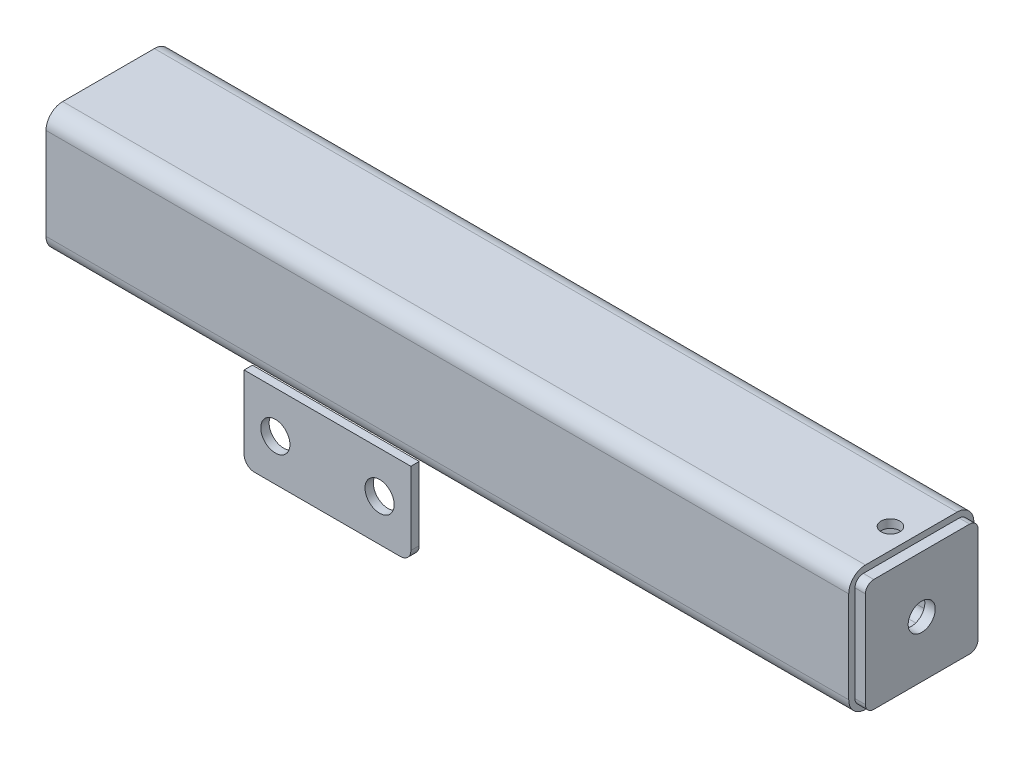
from build123d import *

# Parameters (mm, degrees)
GB_T6728_2002_60_X_60_X_4_1_DEPTH = 385
EXTRUDE_1_DEPTH                   = 5
SKETCH_4_R                        = 7
EXTRUDE_2_DEPTH                   = 4
SKETCH_5_R                        = 6.5
CUT_EXTRUDE_1_DEPTH               = 5


with BuildPart() as part:
    # Sketch1 → 冷弯空心方管gb∕t6728-2002 60 X 60 X 4(1) (new body)
    with BuildSketch(Plane.YZ):
        with BuildLine():
            Line((-22, -30), (22, -30))
            ThreePointArc((22, -30), (27.656854249, -27.656854249), (30, -22))
            Line((30, -22), (30, 22))
            ThreePointArc((30, 22), (27.656854249, 27.656854249), (22, 30))
            Line((22, 30), (-22, 30))
            ThreePointArc((-22, 30), (-27.656854249, 27.656854249), (-30, 22))
            Line((-30, 22), (-30, -22))
            ThreePointArc((-30, -22), (-27.656854249, -27.656854249), (-22, -30))
        make_face()
        with BuildLine():
            Line((-22, -26), (22, -26))
            ThreePointArc((22, -26), (24.828427125, -24.828427125), (26, -22))
            Line((26, -22), (26, 22))
            ThreePointArc((26, 22), (24.828427125, 24.828427125), (22, 26))
            Line((22, 26), (-22, 26))
            ThreePointArc((-22, 26), (-24.828427125, 24.828427125), (-26, 22))
            Line((-26, 22), (-26, -22))
            ThreePointArc((-26, -22), (-24.828427125, -24.828427125), (-22, -26))
        make_face(mode=Mode.SUBTRACT)
    extrude(amount=GB_T6728_2002_60_X_60_X_4_1_DEPTH)

    # 草图8 → M10x1.0 螺纹孔1 (revolve, cut)
    with BuildSketch(Plane(origin=(375, 30, 0), x_dir=(0, 0, 1), z_dir=(1, 0, 0))):
        Polygon((0, 0), (0, 10.703872786), (4.5, 8), (4.5, 0), align=None)
    revolve(axis=Axis((375, 36.35, 0), (0, -1, 0)), mode=Mode.SUBTRACT)


with BuildPart() as body_2:
    # 草图3 → 凸台-拉伸1 (new body)
    with BuildSketch(Plane(origin=(385, 0, 0), x_dir=(0, 0, -1), z_dir=(1, 0, 0))):
        with BuildLine():
            Line((-23, -27), (23, -27))
            ThreePointArc((23, -27), (25.828427125, -25.828427125), (27, -23))
            Line((27, -23), (27, 23))
            ThreePointArc((27, 23), (25.828427125, 25.828427125), (23, 27))
            Line((23, 27), (-23, 27))
            ThreePointArc((-23, 27), (-25.828427125, 25.828427125), (-27, 23))
            Line((-27, 23), (-27, -23))
            ThreePointArc((-27, -23), (-25.828427125, -25.828427125), (-23, -27))
        make_face()
    extrude(amount=EXTRUDE_1_DEPTH)

    # 草图5 → 切除-拉伸1 (cut)
    with BuildSketch(Plane(origin=(390, 0, 0), x_dir=(0, 0, -1), z_dir=(1, 0, 0))):
        Circle(SKETCH_5_R)
    extrude(amount=-CUT_EXTRUDE_1_DEPTH, mode=Mode.SUBTRACT)


with BuildPart() as body_3:
    # 草图4 → 凸台-拉伸2 (new body)
    with BuildSketch(Plane.XY.offset(30)):
        with BuildLine():
            Line((175, -30), (95, -30))
            Line((95, -30), (95, -65))
            ThreePointArc((95, -65), (96.464466094, -68.535533906), (100, -70))
            Line((100, -70), (170, -70))
            ThreePointArc((170, -70), (173.535533906, -68.535533906), (175, -65))
            Line((175, -65), (175, -30))
        make_face()
        with Locations((110, -50)):
            Circle(SKETCH_4_R, mode=Mode.SUBTRACT)
        with Locations((160, -50)):
            Circle(SKETCH_4_R, mode=Mode.SUBTRACT)
    extrude(amount=-EXTRUDE_2_DEPTH)


with BuildPart() as body_4:
    # 镜向2: mirrored copy
    add(body_3.part.mirror(Plane.XY))


solid = Compound([part.part, body_2.part, body_3.part, body_4.part])
